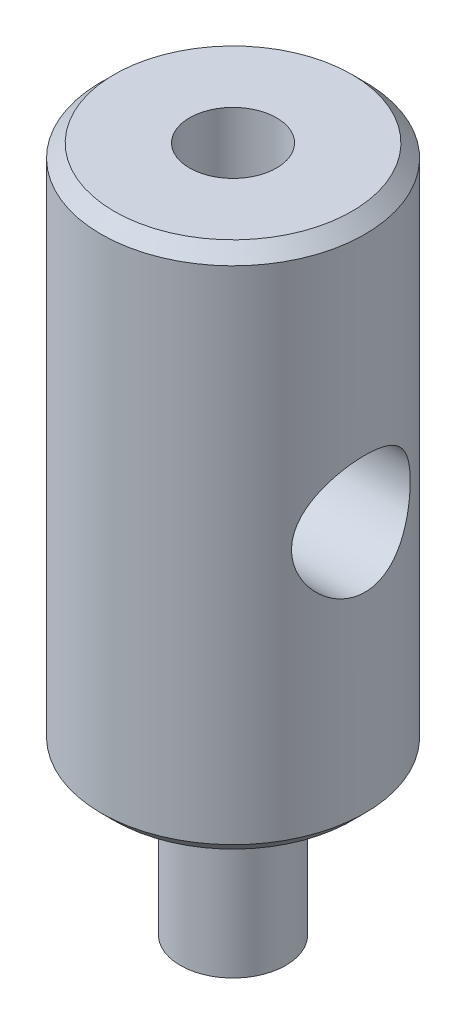
SolidWorks part; units mm, degrees
ref_plane "Front Plane" through (0, 0, 0) normal (0, 0, 1) x (1, 0, 0)
ref_plane "Top Plane" through (0, 0, 0) normal (0, 1, 0) x (1, 0, 0)
ref_plane "Right Plane" through (0, 0, 0) normal (1, 0, 0) x (0, 0, -1)
sketch "Sketch1" plane through (0, 0, 0) normal (0, 1, 0) x (1, 0, 0)
  circle A0 centre (0, 0) radius 5
  dimension "D1" = 10
extrude "Boss-Extrude1" add sketch "Sketch1" along normal mid plane 20
sketch "Sketch2" plane through (0, -10, 0) normal (0, -1, 0) x (1, 0, 0)
  circle A0 centre (0, 0) radius 2
  dimension "D1" = 4
extrude "Boss-Extrude2" add sketch "Sketch2" along normal blind 6
cosmetic thread "Cosmetic Thread1" parameters "D1"=5.5, "D2"=3.3
sketch "Sketch3" plane through (0, 0, 0) normal (0, 0, 1) x (1, 0, 0)
  line L0 (2, -16) -> (2, -10) construction
  line L1 (1.7, -10) -> (2, -10)
  line L2 (1.7, -10) -> (1.7, -10.5)
  line L3 (1.7, -10.5) -> (2, -10.5)
  line L4 (2, -10) -> (2, -10.5)
  line L5 (-2, -10) -> (2, -10) construction
  line L6 (0, 0) -> (0, -26.8399) construction
  dimension "D1" = 0.5
  dimension "D2" = 0.3
revolve "Cut-Revolve1" cut sketch "Sketch3" angle 360 about L6
hole_wizard "M4 Tapped Hole1" positions "Sketch5" profile "Sketch4" tap size "M4" standard "Gb"
sketch "Sketch5" plane through (0, 10, 0) normal (0, 1, 0) x (1, 0, 0)
  point P0 (0, 0)
sketch "Sketch4" plane through (0, 10, 0) normal (1, 0, 0) x (0, 0, 1)
  line L0 (0, 0) -> (0, 11.0914)
  line L1 (0, 11.0914) -> (1.65, 10.1)
  line L2 (1.65, 10.1) -> (1.65, 0)
  line L5 (1.65, 0) -> (0, 0)
  line L10 (0, 11.0914) -> (-1.65, 10.1) construction
  line L11 (0, -6.35) -> (0, 107.95) construction
  dimension "螺纹孔钻头直径" = 3.3
  dimension "螺纹孔钻头深度" = 10.1
  dimension "导头角度" = 118
cosmetic thread "Hole Cosmetic Thread1" parameters "D1"=8, "D2"=4
chamfer "Chamfer1" distance 0.5 angle 45 2 edges at (0, 10, 5) (0, -10, 5)
sketch "Sketch6" plane through (0, 0, 0) normal (1, 0, 0) x (0, 0, -1)
  circle A0 centre (0, 0) radius 2.25
  dimension "D1" = 4.5
extrude "Cut-Extrude1" cut sketch "Sketch6" against normal through all and the other way through all
